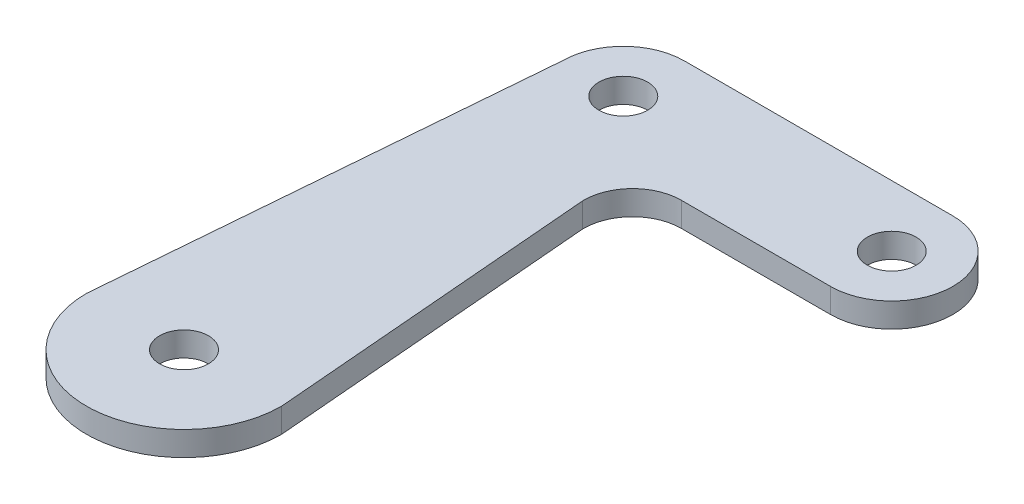
from build123d import *

# Parameters (mm, degrees)
SKETCH1_R           = 3.175
BOSS_EXTRUDE1_DEPTH = 3.175


with BuildPart() as part:
    # Sketch1 → Boss-Extrude1 (new body)
    with BuildSketch(Plane(origin=(0, 0, 0), x_dir=(1, 0, 0), z_dir=(0, 1, 0))):
        with BuildLine():
            Line((0, 7.9502), (34.925, 7.9502))
            ThreePointArc((34.925, 7.9502), (42.8752, 0), (34.925, -7.9502))
            Line((34.925, -7.9502), (15.497902875, -7.9502))
            ThreePointArc((15.497902875, -7.9502), (10.963581061, -9.854705012), (9.149145427, -14.425813956))
            Line((9.149145427, -14.425813956), (12.7, -57.15))
            ThreePointArc((12.7, -57.15), (0, -69.85), (-12.7, -57.15))
            Line((-12.7, -57.15), (-7.9502, 0))
            ThreePointArc((-7.9502, 0), (-5.621640332, 5.621640332), (0, 7.9502))
        make_face()
        with Locations(Location((34.925, 0, 0), (0, 0, 270))):
            Circle(SKETCH1_R, mode=Mode.SUBTRACT)
        with Locations(Location((0, 0, 0), (0, 0, 270))):
            Circle(SKETCH1_R, mode=Mode.SUBTRACT)
        with Locations(Location((0, -57.15, 0), (0, 0, 270))):
            Circle(SKETCH1_R, mode=Mode.SUBTRACT)
    extrude(amount=BOSS_EXTRUDE1_DEPTH)


solid = part.part
